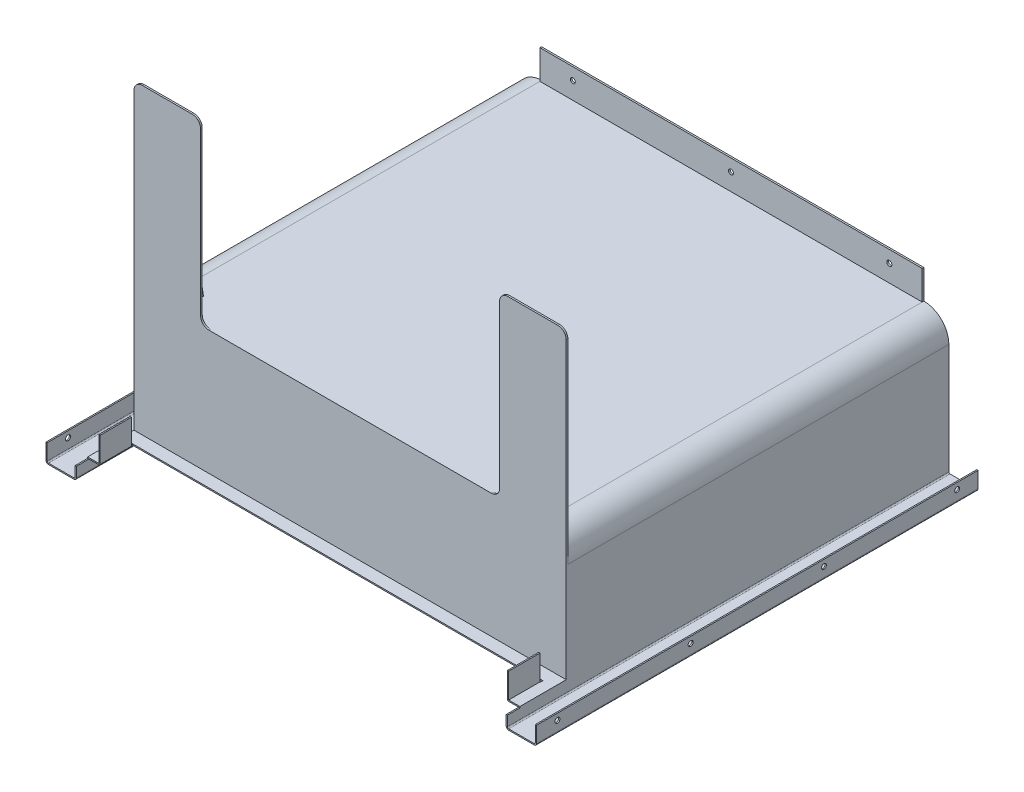
from build123d import *

# Parameters (mm, degrees)
EXTRUDE_1_DEPTH                = 530
FILLET_1_R                     = 3
FILLET_6_R                     = 1.5
SKETCH_2_W                     = 651.298886305
SKETCH_2_H                     = 207.751760279
CUT_EXTRUDE_1_DEPTH            = 72.6
SKETCH_4_W                     = 519
SKETCH_4_H                     = 365
EXTRUDE_10_DEPTH               = 2
SKETCH_5_W                     = 359
SKETCH_5_H                     = 214.5
CUT_EXTRUDE_2_DEPTH            = 622.04014363
FILLET_2_R                     = 10
FILLET_3_R                     = 10
EXTRUDE_13_DEPTH               = 1.5
EXTRUDE_14_DEPTH               = 3
FILLET_4_R                     = 10
SKETCH_13_W                    = 519
SKETCH_13_H                    = 55.6
EXTRUDE_15_DEPTH               = 1.5
SKETCH_14_W                    = 489
SKETCH_14_H                    = 40.6
CUT_EXTRUDE_5_DEPTH            = 1.5
SKETCH_15_W                    = 1.5
SKETCH_15_H                    = 37.6
EXTRUDE_16_DEPTH               = 30
SKETCH_16_W                    = 2
SKETCH_16_H                    = 3
CUT_EXTRUDE_6_DEPTH            = 2
FILLET_5_R                     = 1.5
SKETCH_17_W                    = 459
SKETCH_17_H                    = 35
EXTRUDE_17_DEPTH               = 2
SKETCH_18_W                    = 3
SKETCH_18_H                    = 2
HOLE_WIZARD_6_0_6_1_AT_2_COUNT = 2
HOLE_WIZARD_6_0_6_1_AT_2_PITCH = 190
HOLE_WIZARD_6_0_6_1_AT_3_COUNT = 2
HOLE_WIZARD_6_0_6_1_AT_3_PITCH = 380
SKETCH_20_W                    = 1.5
SKETCH_20_H                    = 7
EXTRUDE_18_DEPTH               = 72.6
HOLE_WIZARD_6_0_6_2_AT_2_COUNT = 2
HOLE_WIZARD_6_0_6_2_AT_2_PITCH = 160
HOLE_WIZARD_6_0_6_2_AT_3_COUNT = 2
HOLE_WIZARD_6_0_6_2_AT_3_PITCH = 320
HOLE_WIZARD_6_0_6_2_AT_4_COUNT = 2
HOLE_WIZARD_6_0_6_2_AT_4_PITCH = 480
HOLE_WIZARD_6_0_6_3_AT_2_COUNT = 2
HOLE_WIZARD_6_0_6_3_AT_2_PITCH = 160
HOLE_WIZARD_6_0_6_3_AT_3_COUNT = 2
HOLE_WIZARD_6_0_6_3_AT_3_PITCH = 320
HOLE_WIZARD_6_0_6_3_AT_4_COUNT = 2
HOLE_WIZARD_6_0_6_3_AT_4_PITCH = 480


with BuildPart() as part:
    # 草图1 → 拉伸-薄壁1 (new body)
    with BuildSketch(Plane.XY):
        with BuildLine():
            Line((293, -61.5), (293, -82))
            Line((293, -82), (261, -82))
            ThreePointArc((261, -82), (259.939339828, -81.560660172), (259.5, -80.5))
            Line((259.5, -80.5), (259.5, 52))
            ThreePointArc((259.5, 52), (250.713203436, 73.213203436), (229.5, 82))
            Line((229.5, 82), (-229.5, 82))
            ThreePointArc((-229.5, 82), (-250.713203436, 73.213203436), (-259.5, 52))
            Line((-259.5, 52), (-259.5, -80.5))
            ThreePointArc((-259.5, -80.5), (-259.939339828, -81.560660172), (-261, -82))
            Line((-261, -82), (-293, -82))
            Line((-293, -82), (-293, -61.5))
            Line((-293, -61.5), (-294.5, -61.5))
            Line((-294.5, -61.5), (-294.5, -83.5))
            Line((-294.5, -83.5), (-261, -83.5))
            ThreePointArc((-261, -83.5), (-258.878679656, -82.621320344), (-258, -80.5))
            Line((-258, -80.5), (-258, 52))
            ThreePointArc((-258, 52), (-249.652543264, 72.152543264), (-229.5, 80.5))
            Line((-229.5, 80.5), (229.5, 80.5))
            ThreePointArc((229.5, 80.5), (249.652543264, 72.152543264), (258, 52))
            Line((258, 52), (258, -80.5))
            ThreePointArc((258, -80.5), (258.878679656, -82.621320344), (261, -83.5))
            Line((261, -83.5), (294.5, -83.5))
            Line((294.5, -83.5), (294.5, -61.5))
            Line((294.5, -61.5), (293, -61.5))
        make_face()
    extrude(amount=EXTRUDE_1_DEPTH)

    # 圆角1
    fillet_1_edges = [part.edges().sort_by_distance(p)[0] for p in [
        (294.5, -83.5, 265),
        (-294.5, -83.5, 265),
    ]]
    fillet(fillet_1_edges, radius=FILLET_1_R)

    # 圆角6
    fillet_6_edges = [part.edges().sort_by_distance(p)[0] for p in [
        (-293, -82, 265),
        (293, -82, 265),
    ]]
    fillet(fillet_6_edges, radius=FILLET_6_R)

    # 草图2 → 切除-拉伸1 (cut)
    with BuildSketch(Plane.XY.offset(530)):
        with Locations((-4.978482744, 35.375880139)):
            Rectangle(SKETCH_2_W, SKETCH_2_H)
    extrude(amount=-CUT_EXTRUDE_1_DEPTH, mode=Mode.SUBTRACT)



with BuildPart() as body_2:
    # 草图4 → 凸台-拉伸10 (new body)
    with BuildSketch(Plane.XY.offset(457.4)):
        with Locations((0, 114)):
            Rectangle(SKETCH_4_W, SKETCH_4_H)
    extrude(amount=EXTRUDE_10_DEPTH)

    # 草图5 → 切除-拉伸2 (cut, through all)
    with BuildSketch(Plane.XY.offset(459.4)):
        with Locations((0, 189.25)):
            Rectangle(SKETCH_5_W, SKETCH_5_H)
    extrude(amount=-CUT_EXTRUDE_2_DEPTH, mode=Mode.SUBTRACT)

    # 圆角2
    fillet_2_edges = [body_2.edges().sort_by_distance(p)[0] for p in [
        (179.5, 82, 458.4),
    ]]
    fillet(fillet_2_edges, radius=FILLET_2_R)

    # 圆角3
    fillet_3_edges = [body_2.edges().sort_by_distance(p)[0] for p in [
        (-179.5, 82, 458.4),
    ]]
    fillet(fillet_3_edges, radius=FILLET_3_R)

    # 圆角4
    fillet_4_edges = [body_2.edges().sort_by_distance(p)[0] for p in [
        (-179.5, 296.5, 458.4),
        (179.5, 296.5, 458.4),
        (-259.5, 296.5, 458.4),
        (259.5, 296.5, 458.4),
    ]]
    fillet(fillet_4_edges, radius=FILLET_4_R)


with BuildPart() as body_3:
    # 草图6 → 凸台-拉伸13 (new, symmetric)
    with BuildSketch(Plane(origin=(-209.5, 0, 0), x_dir=(0, 0, -1), z_dir=(1, 0, 0))):
        Polygon((-457.4, 276.5), (-427.4, 82), (-457.4, 82), align=None)
    extrude(amount=EXTRUDE_13_DEPTH, both=True)


with BuildPart() as body_4:
    # 草图8 → 凸台-拉伸14 (new body)
    with BuildSketch(Plane.ZY.offset(-209.5)):
        Polygon((457.4, 276.5), (427.4, 82), (457.4, 82), align=None)
    extrude(amount=EXTRUDE_14_DEPTH)


with BuildPart() as part_1:
    add(part.part)

    add(body_2.part)  # 凸台-拉伸15 merges body 2
    # 草图13 → 凸台-拉伸15 (add)
    with BuildSketch(Plane(origin=(0, -68.5, 0), x_dir=(1, 0, 0), z_dir=(0, 1, 0))):
        with Locations((0, -487.2)):
            Rectangle(SKETCH_13_W, SKETCH_13_H)
    extrude(amount=EXTRUDE_15_DEPTH)

    # 草图14 → 切除-拉伸5 (cut)
    with BuildSketch(Plane(origin=(0, -67, 0), x_dir=(1, 0, 0), z_dir=(0, 1, 0))):
        with Locations((0, -494.7)):
            Rectangle(SKETCH_14_W, SKETCH_14_H)
    extrude(amount=-CUT_EXTRUDE_5_DEPTH, mode=Mode.SUBTRACT)

    # 草图15 → 凸台-拉伸16 (add)
    with BuildSketch(Plane(origin=(0, -67, 0), x_dir=(1, 0, 0), z_dir=(0, 1, 0))):
        with Locations((245.25, -496.2)):
            Rectangle(SKETCH_15_W, SKETCH_15_H)
        with Locations((-245.25, -496.2)):
            Rectangle(SKETCH_15_W, SKETCH_15_H)
    extrude(amount=EXTRUDE_16_DEPTH)

    # 草图16 → 切除-拉伸6 (cut)
    with BuildSketch(Plane(origin=(0, -67, 0), x_dir=(1, 0, 0), z_dir=(0, 1, 0))):
        with Locations((245.5, -475.9)):
            Rectangle(SKETCH_16_W, SKETCH_16_H)
        with Locations((-245.5, -475.9)):
            Rectangle(SKETCH_16_W, SKETCH_16_H)
    extrude(amount=-CUT_EXTRUDE_6_DEPTH, mode=Mode.SUBTRACT)

    # 圆角5
    fillet_5_edges = [part_1.edges().sort_by_distance(p)[0] for p in [
        (244.5, -68.5, 496.2),
        (-244.5, -68.5, 496.2),
    ]]
    fillet(fillet_5_edges, radius=FILLET_5_R)

    # 草图17 → 凸台-拉伸17 (add)
    with BuildSketch(Plane(origin=(0, 0, 0), x_dir=(-1, 0, 0), z_dir=(0, 0, -1))):
        with Locations((0, 99.5)):
            Rectangle(SKETCH_17_W, SKETCH_17_H)
    extrude(amount=-EXTRUDE_17_DEPTH)

    # 草图18 → Ø6.0 (6) 直径孔1 (revolve, cut)
    with BuildSketch(Plane(origin=(-190, 102.5, 2), x_dir=(0, -1, 0), z_dir=(1, 0, 0))):
        with Locations((1.5, 1)):
            Rectangle(SKETCH_18_W, SKETCH_18_H)
    hole_wizard_6_0_6_1 = revolve(axis=Axis((-190, 102.5, 8.35), (0, 0, -1)), mode=Mode.SUBTRACT)

    # Ø6.0 (6) 直径孔1 at 2: Ø6.0 (6) 直径孔1 ×2
    with Locations(*[(i * HOLE_WIZARD_6_0_6_1_AT_2_PITCH, 0, 0) for i in range(1, HOLE_WIZARD_6_0_6_1_AT_2_COUNT)]):
        add(hole_wizard_6_0_6_1, mode=Mode.SUBTRACT)

    # Ø6.0 (6) 直径孔1 at 3: Ø6.0 (6) 直径孔1 ×2
    with Locations(*[(i * HOLE_WIZARD_6_0_6_1_AT_3_PITCH, 0, 0) for i in range(1, HOLE_WIZARD_6_0_6_1_AT_3_COUNT)]):
        add(hole_wizard_6_0_6_1, mode=Mode.SUBTRACT)

    # 草图20 → 凸台-拉伸18 (add)
    with BuildSketch(Plane.XY.offset(457.4)):
        with Locations((293.75, -65)):
            Rectangle(SKETCH_20_W, SKETCH_20_H)
        with Locations((-293.75, -65)):
            Rectangle(SKETCH_20_W, SKETCH_20_H)
    extrude(amount=EXTRUDE_18_DEPTH)

    # 草图21 → Ø6.0 (6) 直径孔2 (revolve, cut)
    with BuildSketch(Plane(origin=(294.5, -69, 505), x_dir=(0, 0, -1), z_dir=(0, 1, 0))):
        Polygon((0, 0), (0, 3.802581857), (3, 2), (3, 0), align=None)
    hole_wizard_6_0_6_2 = revolve(axis=Axis((300.85, -69, 505), (-1, 0, 0)), mode=Mode.SUBTRACT)

    # Ø6.0 (6) 直径孔2 at 2: Ø6.0 (6) 直径孔2 ×2
    with Locations(*[(0, 0, -i * HOLE_WIZARD_6_0_6_2_AT_2_PITCH) for i in range(1, HOLE_WIZARD_6_0_6_2_AT_2_COUNT)]):
        add(hole_wizard_6_0_6_2, mode=Mode.SUBTRACT)

    # Ø6.0 (6) 直径孔2 at 3: Ø6.0 (6) 直径孔2 ×2
    with Locations(*[(0, 0, -i * HOLE_WIZARD_6_0_6_2_AT_3_PITCH) for i in range(1, HOLE_WIZARD_6_0_6_2_AT_3_COUNT)]):
        add(hole_wizard_6_0_6_2, mode=Mode.SUBTRACT)

    # Ø6.0 (6) 直径孔2 at 4: Ø6.0 (6) 直径孔2 ×2
    with Locations(*[(0, 0, -i * HOLE_WIZARD_6_0_6_2_AT_4_PITCH) for i in range(1, HOLE_WIZARD_6_0_6_2_AT_4_COUNT)]):
        add(hole_wizard_6_0_6_2, mode=Mode.SUBTRACT)

    # 草图23 → Ø6.0 (6) 直径孔3 (revolve, cut)
    with BuildSketch(Plane(origin=(-294.5, -69, 25), x_dir=(0, 0, 1), z_dir=(0, 1, 0))):
        Polygon((0, 0), (0, 3.802581857), (3, 2), (3, 0), align=None)
    hole_wizard_6_0_6_3 = revolve(axis=Axis((-300.85, -69, 25), (1, 0, 0)), mode=Mode.SUBTRACT)

    # Ø6.0 (6) 直径孔3 at 2: Ø6.0 (6) 直径孔3 ×2
    with Locations(*[(0, 0, i * HOLE_WIZARD_6_0_6_3_AT_2_PITCH) for i in range(1, HOLE_WIZARD_6_0_6_3_AT_2_COUNT)]):
        add(hole_wizard_6_0_6_3, mode=Mode.SUBTRACT)

    # Ø6.0 (6) 直径孔3 at 3: Ø6.0 (6) 直径孔3 ×2
    with Locations(*[(0, 0, i * HOLE_WIZARD_6_0_6_3_AT_3_PITCH) for i in range(1, HOLE_WIZARD_6_0_6_3_AT_3_COUNT)]):
        add(hole_wizard_6_0_6_3, mode=Mode.SUBTRACT)

    # Ø6.0 (6) 直径孔3 at 4: Ø6.0 (6) 直径孔3 ×2
    with Locations(*[(0, 0, i * HOLE_WIZARD_6_0_6_3_AT_4_PITCH) for i in range(1, HOLE_WIZARD_6_0_6_3_AT_4_COUNT)]):
        add(hole_wizard_6_0_6_3, mode=Mode.SUBTRACT)


solid = Compound([body_3.part, body_4.part, part_1.part])
